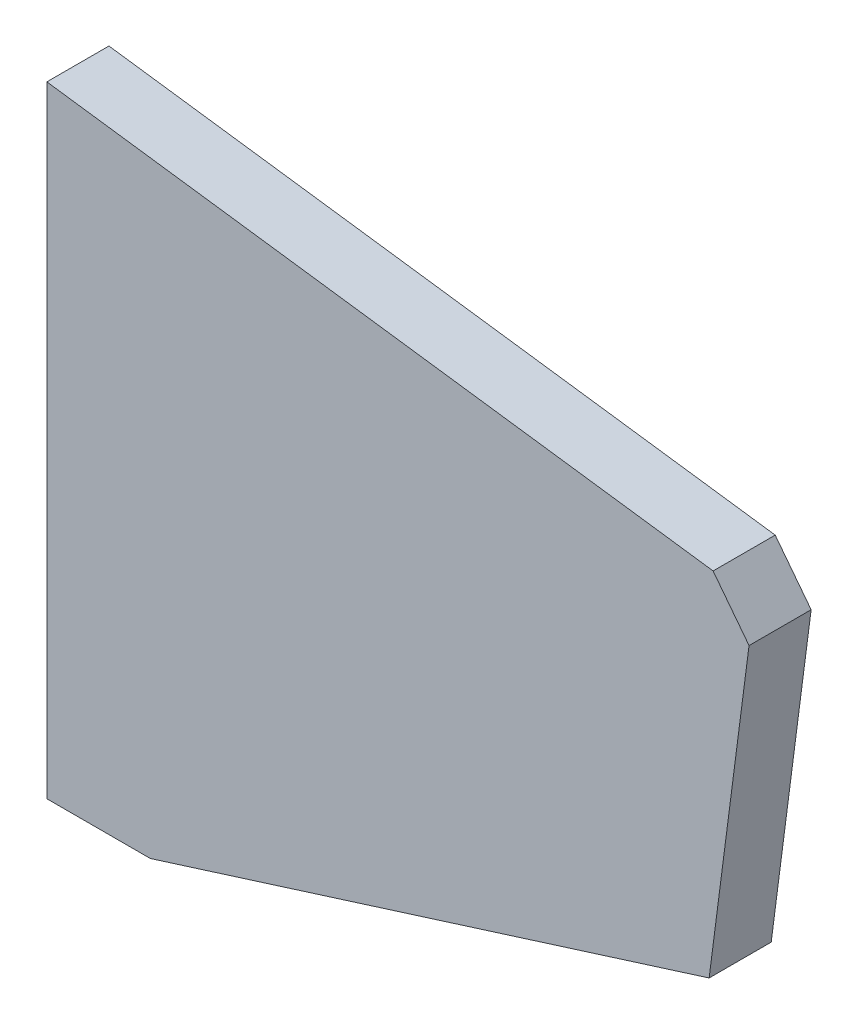
SolidWorks part; units mm, degrees
material "1023 碳钢板 (SS)"
ref_plane "Front Plane" through (0, 0, 0) normal (0, 0, 1) x (1, 0, 0)
ref_plane "Top Plane" through (0, 0, 0) normal (0, 1, 0) x (1, 0, 0)
ref_plane "Right Plane" through (0, 0, 0) normal (1, 0, 0) x (0, 0, -1)
sketch "Sketch1" plane through (0, 0, 0) normal (0, 0, 1) x (1, 0, 0)
  line L0 (0, 0) -> (0, 60)
  line L1 (0, 60) -> (68.3729, 50.7182)
  line L3 (64, 17) -> (10, 0)
  line L4 (10, 0) -> (0, 0)
  line L5 (68.3729, 50.7182) -> (64, 17)
  dimension "D1" = 69
  dimension "D2" = 34
  dimension "D3" = 10
  dimension "D4" = 17
  dimension "D5" = 54
  dimension "D6" = 60
extrude "Boss-Extrude1" add sketch "Sketch1" along normal blind 6 contours L5 L3 L4 L0 L1
chamfer "Chamfer1" distance 4 angle 45 1 edges at (68.3729, 50.7182, 3)
